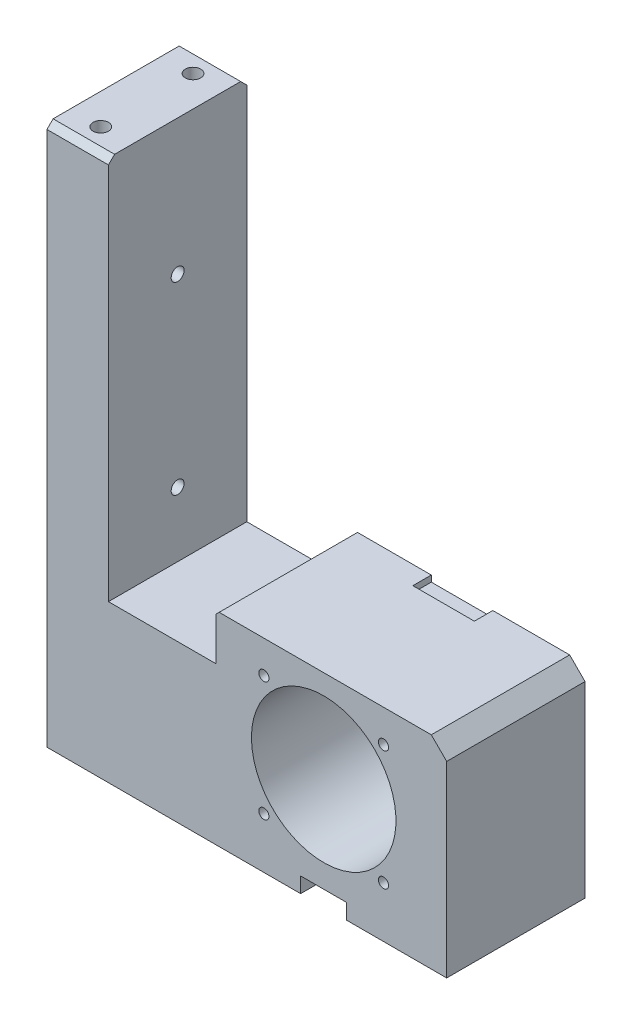
from build123d import *

# Parameters (mm, degrees)
SKETCH1_R             = 23.5
BOSS_EXTRUDE1_DEPTH   = 45
M6_TAPPED_HOLE1_D     = 5
M6_TAPPED_HOLE1_DEPTH = 15
M6_TAPPED_HOLE1_TIP   = 1.502151548
M5_TAPPED_HOLE1_D     = 4.2
M6_TAPPED_HOLE2_D     = 5
M6_TAPPED_HOLE2_DEPTH = 15
M6_TAPPED_HOLE2_TIP   = 1.502151548
M4_TAPPED_HOLE1_D     = 3.3
M4_TAPPED_HOLE1_DEPTH = 10.1
M4_TAPPED_HOLE1_TIP   = 0.991420021
CHAMFER1_SIZE         = 5
CHAMFER2_SIZE         = 2
SKETCH15_W            = 35
SKETCH15_H            = 15
CUT_EXTRUDE1_DEPTH    = 173.409396496
CHAMFER3_SIZE         = 1
SKETCH18_W            = 20
SKETCH18_H            = 6
CUT_EXTRUDE2_DEPTH    = 2


with BuildPart() as part:
    # Sketch1 → Boss-Extrude1 (new body)
    with BuildSketch(Plane.XY):
        Polygon((-90, 140), (-90, -36), (-7.5, -36), (-7.5, -31), (7.5, -31), (7.5, -36), (40, -36), (40, 30), (-70, 30), (-70, 140), align=None)
        with Locations(Location((0, 0, 0), (0, 0, 180))):
            Circle(SKETCH1_R, mode=Mode.SUBTRACT)
    extrude(amount=BOSS_EXTRUDE1_DEPTH)

    # M6 Tapped Hole1
    with Locations(Plane.XZ.offset(36)):
        with Locations((-75, 8), (25, 8), (-75, 26), (25, 26)):
            Hole(M6_TAPPED_HOLE1_D / 2, depth=M6_TAPPED_HOLE1_DEPTH)
            with Locations((0, 0, -(M6_TAPPED_HOLE1_DEPTH + M6_TAPPED_HOLE1_TIP / 2))):  # 118° drill point
                Cone(0, M6_TAPPED_HOLE1_D / 2, M6_TAPPED_HOLE1_TIP, mode=Mode.SUBTRACT)

    # M5 Tapped Hole1 (through all)
    with Locations(Plane(origin=(-70, 0, 0), x_dir=(0, 0, -1), z_dir=(1, 0, 0))):
        with Locations((-22.5, 96), (-22.5, 36)):
            Hole(M5_TAPPED_HOLE1_D / 2)

    # M6 Tapped Hole2
    with Locations(Plane(origin=(0, 140, 0), x_dir=(-1, 0, 0), z_dir=(0, 1, 0))):
        with Locations((80, 7.5), (80, 37.5)):
            Hole(M6_TAPPED_HOLE2_D / 2, depth=M6_TAPPED_HOLE2_DEPTH)
            with Locations((0, 0, -(M6_TAPPED_HOLE2_DEPTH + M6_TAPPED_HOLE2_TIP / 2))):  # 118° drill point
                Cone(0, M6_TAPPED_HOLE2_D / 2, M6_TAPPED_HOLE2_TIP, mode=Mode.SUBTRACT)

    # M4 Tapped Hole1
    with Locations(Plane.XY.offset(45)):
        with Locations((-19.445436483, -19.445436483), (19.445436483, -19.445436483), (19.445436483, 19.445436483), (-19.445436483, 19.445436483)):
            Hole(M4_TAPPED_HOLE1_D / 2, depth=M4_TAPPED_HOLE1_DEPTH)
            with Locations((0, 0, -(M4_TAPPED_HOLE1_DEPTH + M4_TAPPED_HOLE1_TIP / 2))):  # 118° drill point
                Cone(0, M4_TAPPED_HOLE1_D / 2, M4_TAPPED_HOLE1_TIP, mode=Mode.SUBTRACT)

    # Chamfer1
    chamfer1_edges = [part.edges().sort_by_distance(p)[0] for p in [
        (40, 30, 22.5),
    ]]
    chamfer(chamfer1_edges, length=CHAMFER1_SIZE)

    # Chamfer2
    chamfer2_edges = [part.edges().sort_by_distance(p)[0] for p in [
        (-80, 140, 45),
        (-80, 140, 0),
    ]]
    chamfer(chamfer2_edges, length=CHAMFER2_SIZE)

    # Sketch15 → Cut-Extrude1 (cut, through all)
    with BuildSketch(Plane.XY.offset(45)):
        with Locations((-52.5, 22.5)):
            Rectangle(SKETCH15_W, SKETCH15_H)
    extrude(amount=-CUT_EXTRUDE1_DEPTH, mode=Mode.SUBTRACT)

    # Chamfer3
    chamfer3_edges = [part.edges().sort_by_distance(p)[0] for p in [
        (-35, 30, 22.5),
    ]]
    chamfer(chamfer3_edges, length=CHAMFER3_SIZE)

    # Sketch18 → Cut-Extrude2 (cut)
    with BuildSketch(Plane(origin=(0, 30, 0), x_dir=(1, 0, 0), z_dir=(0, 1, 0))):
        with Locations((0, -3)):
            Rectangle(SKETCH18_W, SKETCH18_H)
    extrude(amount=-CUT_EXTRUDE2_DEPTH, mode=Mode.SUBTRACT)


solid = part.part
